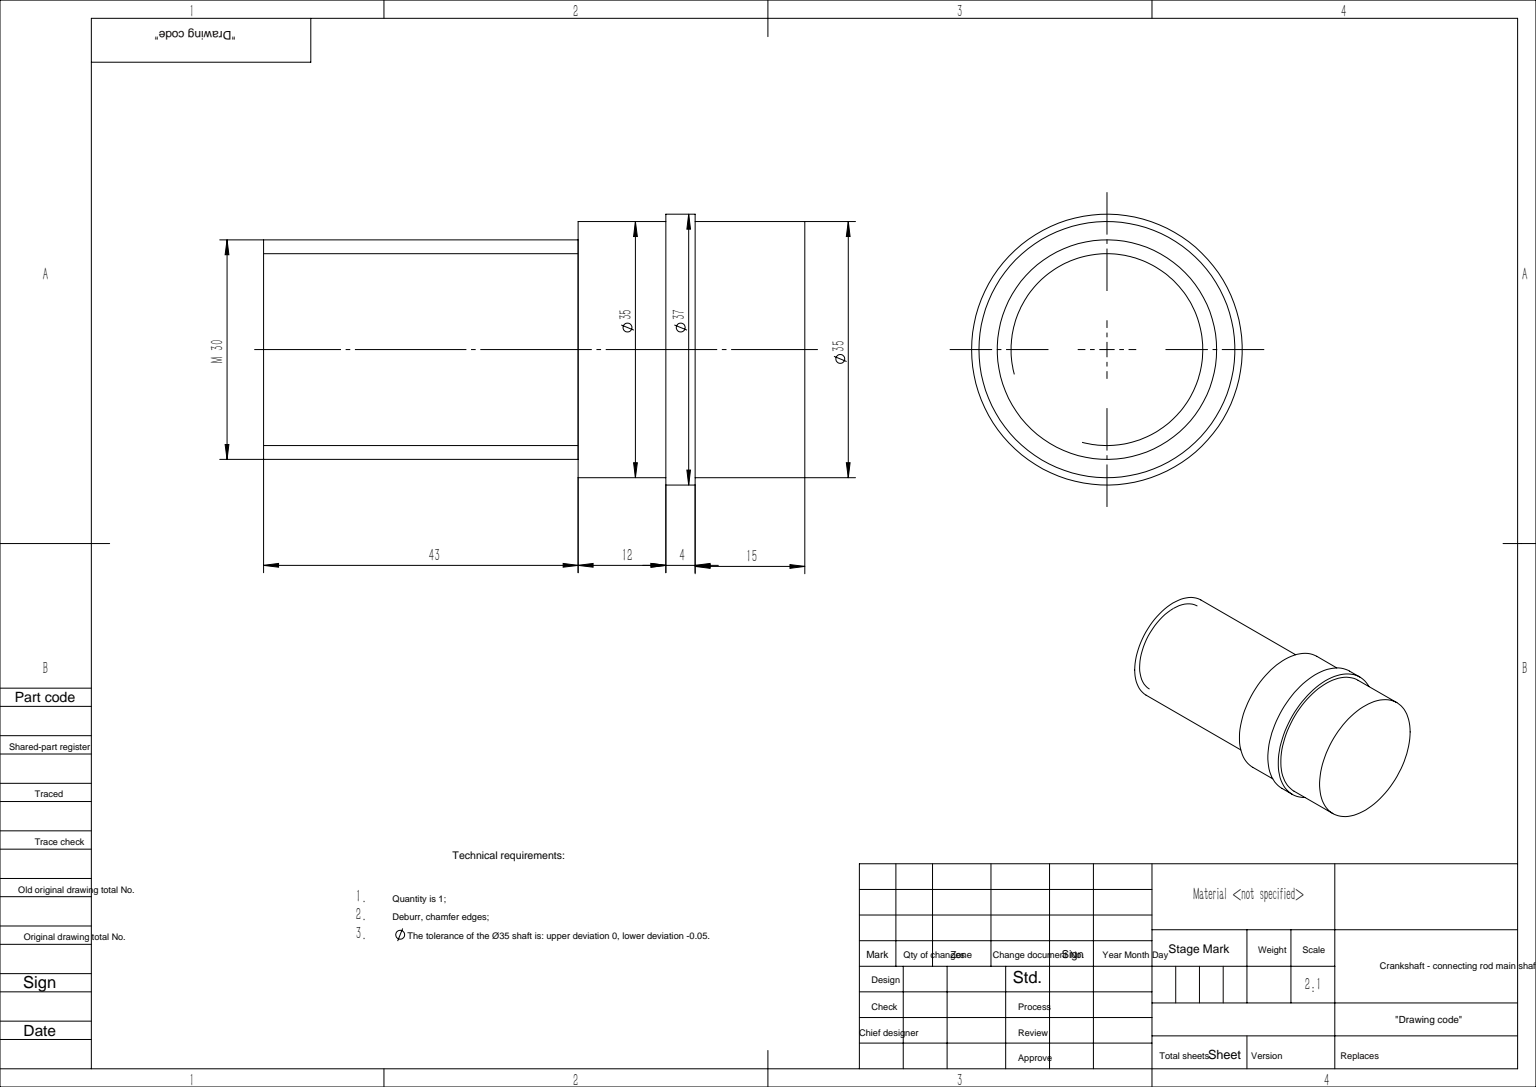
from build123d import *

# Parameters (mm, degrees)
SKETCH_1_R      = 17.5
EXTRUDE_1_DEPTH = 31
SKETCH_2_R      = 15
EXTRUDE_2_DEPTH = 43
SKETCH_4_R      = 18.5
EXTRUDE_3_DEPTH = 4


with BuildPart() as part:
    # 草图1 → 凸台-拉伸1 (new body)
    with BuildSketch(Plane(origin=(0, 0, 0), x_dir=(0, 0, -1), z_dir=(1, 0, 0))):
        Circle(SKETCH_1_R)
    extrude(amount=EXTRUDE_1_DEPTH)

    # 草图2 → 凸台-拉伸2 (add)
    with BuildSketch(Plane.ZY):
        with Locations(Location((0, 0, 0), (0, 0, 180))):
            Circle(SKETCH_2_R)
    extrude(amount=EXTRUDE_2_DEPTH)

    # 草图4 → 凸台-拉伸3 (add)
    with BuildSketch(Plane(origin=(12, 0, 0), x_dir=(0, 0, -1), z_dir=(1, 0, 0))):
        Circle(SKETCH_4_R)
    extrude(amount=EXTRUDE_3_DEPTH)


solid = part.part
